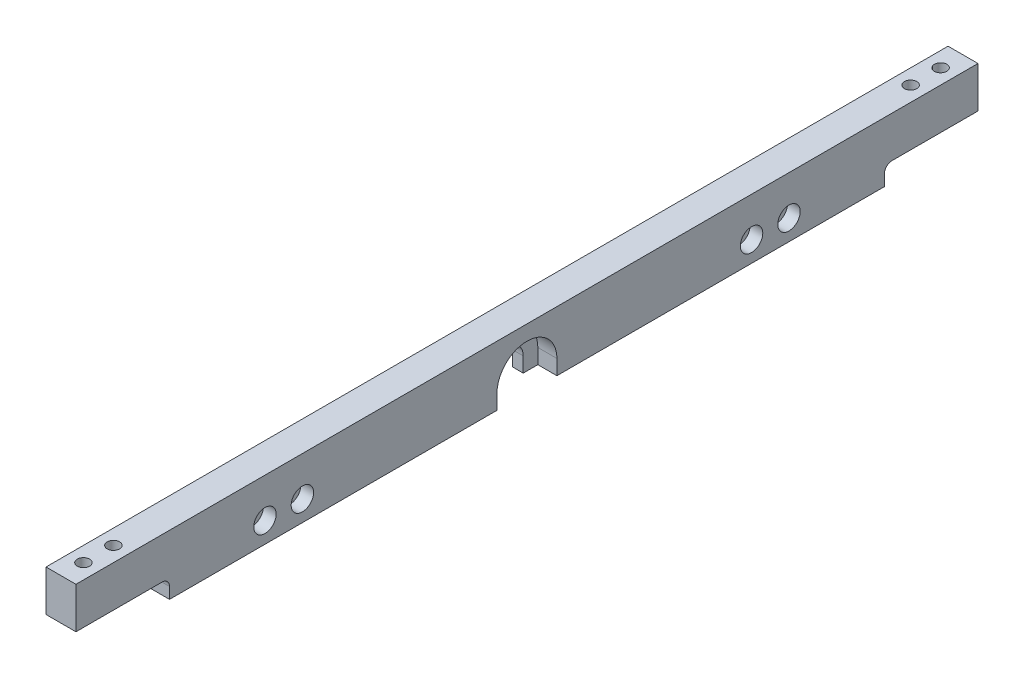
from build123d import *

# Parameters (mm, degrees)
SKETCH3_W                                            = 8
SKETCH3_H                                            = 16
BOSS_EXTRUDE2_DEPTH                                  = 241
CUT_EXTRUDE1_DEPTH                                   = 5.1
CUT_EXTRUDE2_DEPTH                                   = 242.584374495
CBORE_FOR_M3_HEXAGON_SOCKET_HEAD_CAP_SCR_D           = 3.4
CBORE_FOR_M3_HEXAGON_SOCKET_HEAD_CAP_SCR_DEPTH       = 10.1
CBORE_FOR_M3_HEXAGON_SOCKET_HEAD_CAP_SCR_CBORE_D     = 6
CBORE_FOR_M3_HEXAGON_SOCKET_HEAD_CAP_SCR_CBORE_DEPTH = 3.4
CBORE_FOR_M3_HEXAGON_SOCKET_HEAD_CAP_SCR_TIP         = 1.021463052
M4_TAPPED_HOLE1_D                                    = 3.3
M4_TAPPED_HOLE1_DEPTH                                = 9.1
M4_TAPPED_HOLE1_TIP                                  = 0.991420021
CUT_EXTRUDE3_DEPTH                                   = 242.662988478


with BuildPart() as part:
    # Sketch3 → Boss-Extrude2 (new body)
    with BuildSketch(Plane.XY):
        with Locations((4, 8)):
            Rectangle(SKETCH3_W, SKETCH3_H)
    extrude(amount=BOSS_EXTRUDE2_DEPTH)

    # Sketch4 → Cut-Extrude1 (cut)
    with BuildSketch(Plane(origin=(8, 0, 0), x_dir=(0, 0, -1), z_dir=(1, 0, 0))):
        with BuildLine():
            Line((-112.5, 4), (-112.5, 0))
            ThreePointArc((-112.5, 0), (-120.5, -8), (-128.5, 0))
            Line((-128.5, 0), (-128.5, 4))
            ThreePointArc((-128.5, 4), (-120.5, 12), (-112.5, 4))
        make_face()
    extrude(amount=-CUT_EXTRUDE1_DEPTH, mode=Mode.SUBTRACT)

    # Sketch5 → Cut-Extrude2 (cut, through all)
    with BuildSketch(Plane(origin=(2.9, 0, 0), x_dir=(0, 0, -1), z_dir=(1, 0, 0))):
        with BuildLine():
            Line((-116.4, 4), (-116.4, 0))
            ThreePointArc((-116.4, 0), (-120.5, -4.1), (-124.6, 0))
            Line((-124.6, 0), (-124.6, 4))
            ThreePointArc((-124.6, 4), (-120.5, 8.1), (-116.4, 4))
        make_face()
    extrude(amount=-CUT_EXTRUDE2_DEPTH, mode=Mode.SUBTRACT)

    # CBORE for M3 Hexagon socket head cap screws1
    with Locations(Plane(origin=(8, 0, 0), x_dir=(0, 0, -1), z_dir=(1, 0, 0))):
        with Locations((-60.5, 5.5), (-50.5, 5.5), (-190.5, 5.5), (-180.5, 5.5)):
            CounterBoreHole(CBORE_FOR_M3_HEXAGON_SOCKET_HEAD_CAP_SCR_D / 2, CBORE_FOR_M3_HEXAGON_SOCKET_HEAD_CAP_SCR_CBORE_D / 2, CBORE_FOR_M3_HEXAGON_SOCKET_HEAD_CAP_SCR_CBORE_DEPTH, depth=CBORE_FOR_M3_HEXAGON_SOCKET_HEAD_CAP_SCR_DEPTH)
            with Locations((0, 0, -(CBORE_FOR_M3_HEXAGON_SOCKET_HEAD_CAP_SCR_DEPTH + CBORE_FOR_M3_HEXAGON_SOCKET_HEAD_CAP_SCR_TIP / 2))):  # 118° drill point
                Cone(0, CBORE_FOR_M3_HEXAGON_SOCKET_HEAD_CAP_SCR_D / 2, CBORE_FOR_M3_HEXAGON_SOCKET_HEAD_CAP_SCR_TIP, mode=Mode.SUBTRACT)

    # M4 Tapped Hole1
    with Locations(Plane(origin=(0, 16, 0), x_dir=(1, 0, 0), z_dir=(0, 1, 0))):
        with Locations((4, -235), (4, -227), (4, -14), (4, -6)):
            Hole(M4_TAPPED_HOLE1_D / 2, depth=M4_TAPPED_HOLE1_DEPTH)
            with Locations((0, 0, -(M4_TAPPED_HOLE1_DEPTH + M4_TAPPED_HOLE1_TIP / 2))):  # 118° drill point
                Cone(0, M4_TAPPED_HOLE1_D / 2, M4_TAPPED_HOLE1_TIP, mode=Mode.SUBTRACT)

    # Sketch10 → Cut-Extrude3 (cut, through all)
    with BuildSketch(Plane(origin=(8, 0, 0), x_dir=(0, 0, -1), z_dir=(1, 0, 0))):
        with BuildLine():
            Line((0, 0), (-25, 0))
            Line((-25, 0), (-25, 3))
            ThreePointArc((-25, 3), (-24.414213562, 4.414213562), (-23, 5))
            Line((-23, 5), (0, 5))
            Line((0, 5), (0, 0))
        make_face()
        with BuildLine():
            Line((-216, 0), (-216, 3))
            ThreePointArc((-216, 3), (-216.585786438, 4.414213562), (-218, 5))
            Line((-218, 5), (-241, 5))
            Line((-241, 5), (-241, 0))
            Line((-241, 0), (-216, 0))
        make_face()
    extrude(amount=-CUT_EXTRUDE3_DEPTH, mode=Mode.SUBTRACT)


solid = part.part
